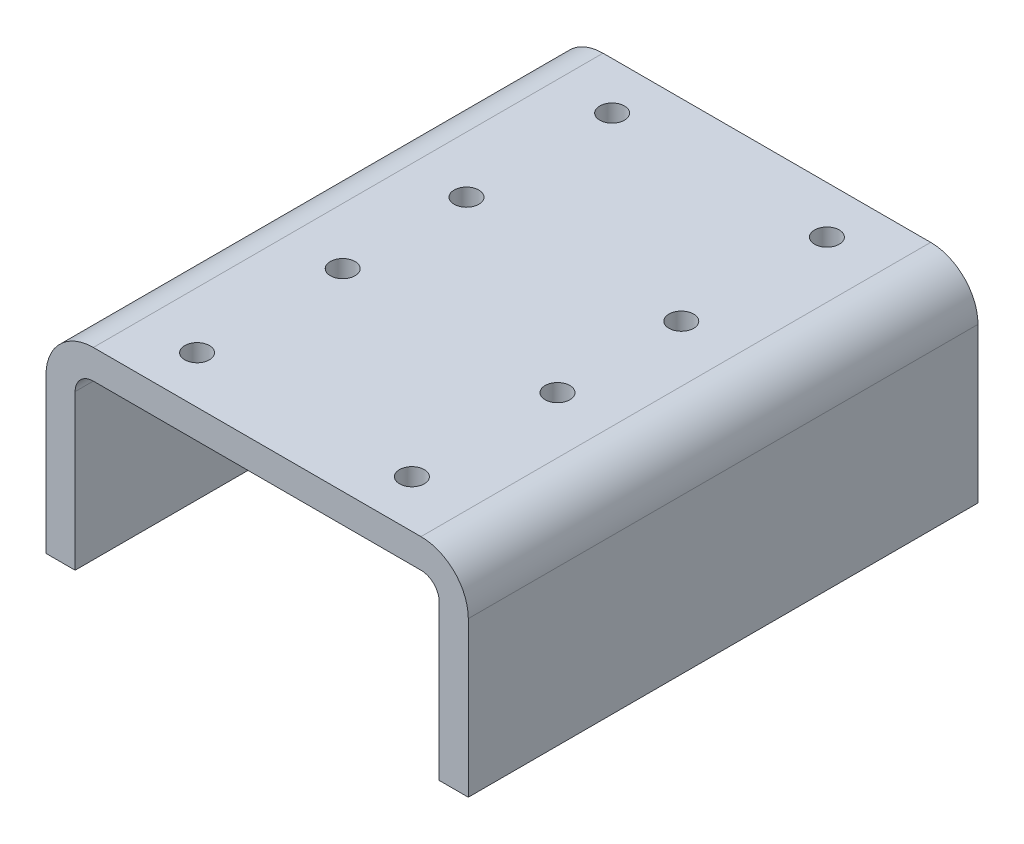
from build123d import *

# Parameters (mm, degrees)
BOSS_EXTRUDE1_DEPTH   = 140
M8_TAPPED_HOLE1_D     = 6.8
M8_TAPPED_HOLE1_DEPTH = 19.75
M8_TAPPED_HOLE1_TIP   = 2.042926105


with BuildPart() as part:
    # Sketch1 → Boss-Extrude1 (new body)
    with BuildSketch(Plane.XY):
        with BuildLine():
            Line((0, 0), (0, 42.5))
            ThreePointArc((0, 42.5), (3.807611845, 51.692388155), (13, 55.5))
            Line((13, 55.5), (103, 55.5))
            ThreePointArc((103, 55.5), (112.192388155, 51.692388155), (116, 42.5))
            Line((116, 42.5), (116, 0))
            Line((116, 0), (108, 0))
            Line((108, 0), (108, 42.5))
            ThreePointArc((108, 42.5), (106.535533906, 46.035533906), (103, 47.5))
            Line((103, 47.5), (13, 47.5))
            ThreePointArc((13, 47.5), (9.464466094, 46.035533906), (8, 42.5))
            Line((8, 42.5), (8, 0))
            Line((8, 0), (0, 0))
        make_face()
    extrude(amount=BOSS_EXTRUDE1_DEPTH)

    # M8 Tapped Hole1
    with Locations(Plane(origin=(0, 55.5, 0), x_dir=(1, 0, 0), z_dir=(0, 1, 0))):
        with Locations((28.5, -13), (87.5, -13), (87.5, -53), (28.5, -53), (28.5, -87), (87.5, -87), (87.5, -127), (28.5, -127)):
            Hole(M8_TAPPED_HOLE1_D / 2, depth=M8_TAPPED_HOLE1_DEPTH)
            with Locations((0, 0, -(M8_TAPPED_HOLE1_DEPTH + M8_TAPPED_HOLE1_TIP / 2))):  # 118° drill point
                Cone(0, M8_TAPPED_HOLE1_D / 2, M8_TAPPED_HOLE1_TIP, mode=Mode.SUBTRACT)


solid = part.part
